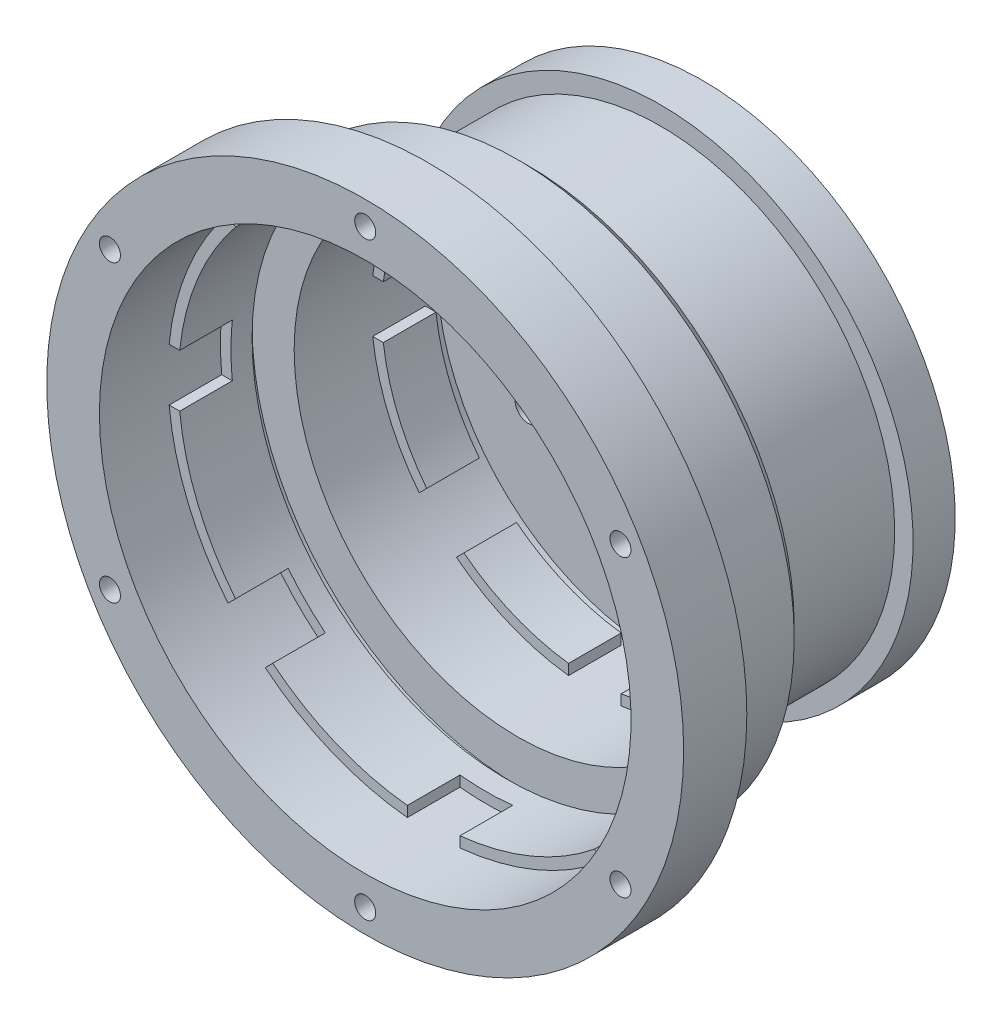
SolidWorks part; units mm, degrees
material "HT200"
ref_plane "Front Plane" through (0, 0, 0) normal (0, 0, 1) x (1, 0, 0)
ref_plane "Top Plane" through (0, 0, 0) normal (0, 1, 0) x (1, 0, 0)
ref_plane "Right Plane" through (0, 0, 0) normal (1, 0, 0) x (0, 0, -1)
other "Configuration Table"
sketch "Sketch1" plane through (0, 0, 0) normal (0, 1, 0) x (1, 0, 0)
  line L0 (0, 60) -> (0, 0) construction
  line L1 (50.5, 3.9057) -> (50.5, 16.9057)
  line L2 (50.5, 32.9057) -> (42.5, 32.9057)
  line L3 (42.5, 32.9057) -> (42.5, 47.5353)
  line L5 (44.5, 34.9057) -> (44.5, 62) construction
  line L6 (52.5, 3.9057) -> (52.5, 34.9057)
  line L7 (52.5, 34.9057) -> (44.5, 34.9057)
  line L8 (44.5, 34.9057) -> (44.5, 60)
  line L9 (52.5, 3.9057) -> (50.5, 3.9057)
  line L10 (42.5, 60) -> (44.5, 60)
  line L12 (42.5, 60) -> (0, 60) construction
  line L13 (44.5, 62) -> (0, 62) construction
  line L16 (-50, 5.9057) -> (50, 5.9057) construction
  line L17 (42.5, 47.5353) -> (40.5, 47.5353)
  line L18 (40.5, 47.5353) -> (40.5, 57.5353)
  line L19 (40.5, 57.5353) -> (42.5, 57.5353)
  line L20 (42, 57.5353) -> (39.6863, 57.5353) construction
  line L21 (42, 47.5353) -> (39.6863, 47.5353) construction
  line L22 (42.5, 57.5353) -> (42.5, 60)
  line L23 (42.5, 32.9057) -> (42.5, 60) construction
  line L24 (50.5, 30.9057) -> (48.5, 30.9057)
  line L25 (47.7389, 30.9057) -> (37.292, 30.9057) construction
  line L26 (48.5, 30.9057) -> (48.5, 16.9057)
  line L30 (50.5, 30.9057) -> (50.5, 32.9057)
  line L31 (50.5, 3.9057) -> (50.5, 32.9057) construction
  line L33 (48.5, 16.9057) -> (50.5, 16.9057)
  line L34 (47.7389, 16.9057) -> (50, 16.9057) construction
  dimension "D1" = 50.5
  dimension "D2" = 42.5
  dimension "D3" = 2
  dimension "D4" = 2
  dimension "D6" = 2
  dimension "D7" = 2
  dimension "D5" = 2
revolve "Revolve1" add sketch "Sketch1" angle 360 about L0
sketch "Sketch2" plane through (0, 0, -16.9057) normal (0, 0, 1) x (1, 0, 0)
  line L0 (0, 7.0428) -> (0, -3.6627) construction
  line L7 (-5, 50.2519) -> (-5, 48.2416)
  line L9 (5, 50.2519) -> (5, 48.2416)
  circle A0 centre (0, 0) radius 48.5 construction
  circle A1 centre (0, 0) radius 48.5
  circle A4 centre (0, 0) radius 50.5
  circle A5 centre (0, 0) radius 50.5
  circle M11 centre (0, 0) radius 50.5
  circle M12 centre (0, 0) radius 48.5
  dimension "D2" = 0
sketch "Sketch3" plane through (0, 0, -47.5353) normal (0, 0, 1) x (1, 0, 0)
  line L0 (0, 5.1524) -> (0, -5.1598) construction
  line L2 (-5, 42.2049) -> (-5, 40.1902)
  line L4 (5, 42.2049) -> (5, 40.1902)
  line L5 (33.3789, 26.3078) -> (31.9543, 24.8832)
  line L6 (26.3078, 33.3789) -> (24.8832, 31.9543)
  line L7 (42.2049, -5) -> (40.1902, -5)
  line L8 (42.2049, 5) -> (40.1902, 5)
  line L9 (26.3078, -33.3789) -> (24.8832, -31.9543)
  line L10 (33.3789, -26.3078) -> (31.9543, -24.8832)
  line L11 (-5, -42.2049) -> (-5, -40.1902)
  line L12 (5, -42.2049) -> (5, -40.1902)
  line L13 (-33.3789, -26.3078) -> (-31.9543, -24.8832)
  line L14 (-26.3078, -33.3789) -> (-24.8832, -31.9543)
  line L15 (-42.2049, 5) -> (-40.1902, 5)
  line L16 (-42.2049, -5) -> (-40.1902, -5)
  line L17 (-26.3078, 33.3789) -> (-24.8832, 31.9543)
  line L18 (-33.3789, 26.3078) -> (-31.9543, 24.8832)
  circle A0 centre (0, 0) radius 40.5 construction
  circle A1 centre (0, 0) radius 42.5
  circle A2 centre (0, 0) radius 42.5
  circle A3 centre (0, 0) radius 40.5
  point P43 (0, 0)
  circle M6 centre (0, 0) radius 42.5
  circle M7 centre (0, 0) radius 40.5
  dimension "D2" = 8
  dimension "D1" = 0
extrude "Cut-Extrude2" cut sketch "Sketch3" against normal blind 10 contours L4 L2 M6 M7 | L6 L5 M6 M7 | L8 L7 M6 M7 | L10 L9 M6 M7 | L12 L11 M6 M7 | L14 L13 M6 M7 | L16 L15 M6 M7 | L18 L17 M6 M7 | A3
extrude "Cut-Extrude3" cut sketch "Sketch2" against normal blind 10 contours L9 L7 M11 M12
pattern_circular "CirPattern5" count 8 over 360 about axis through (0, 0, 0) along (0, 0, 1) of "Cut-Extrude3"
chamfer "Chamfer1" distance 2 angle 45 1 edges at (-52.5, 0, -34.9057)
sketch "Sketch4" plane through (0, 0, -60) normal (0, 0, -1) x (-1, 0, 0)
  circle A0 centre (0, 0) radius 48
  circle A1 centre (0, 0) radius 15
  circle A3 centre (0, 0) radius 29 construction
  circle A4 centre (0, 29) radius 2.5
  circle A5 centre (25.1147, 14.5) radius 2.5
  circle A6 centre (25.1147, -14.5) radius 2.5
  circle A7 centre (0, -29) radius 2.5
  circle A8 centre (-25.1147, -14.5) radius 2.5
  circle A9 centre (-25.1147, 14.5) radius 2.5
  point P19 (0, 0)
  dimension "D1" = 96
  dimension "D2" = 30
  dimension "D3" = 58
  dimension "D4" = 5
  dimension "D5" = 6
extrude "Boss-Extrude1" add sketch "Sketch4" along normal blind 8
sketch "Sketch7" plane through (0, 0, -3.9057) normal (0, 0, 1) x (1, 0, 0)
  circle A0 centre (0, 0) radius 52.5
  circle A1 centre (0, 0) radius 60.5
  circle A2 centre (0, 0) radius 56 construction
  circle A3 centre (0, 56) radius 2
  circle A4 centre (48.4974, 28) radius 2
  circle A5 centre (48.4974, -28) radius 2
  circle A6 centre (0, -56) radius 2
  circle A7 centre (-48.4974, -28) radius 2
  circle A8 centre (-48.4974, 28) radius 2
  point P20 (0, 0)
  dimension "D2" = 112
  dimension "D3" = 4
  dimension "D1" = 8
  dimension "D4" = 6
extrude "Boss-Extrude2" add sketch "Sketch7" against normal blind 12
